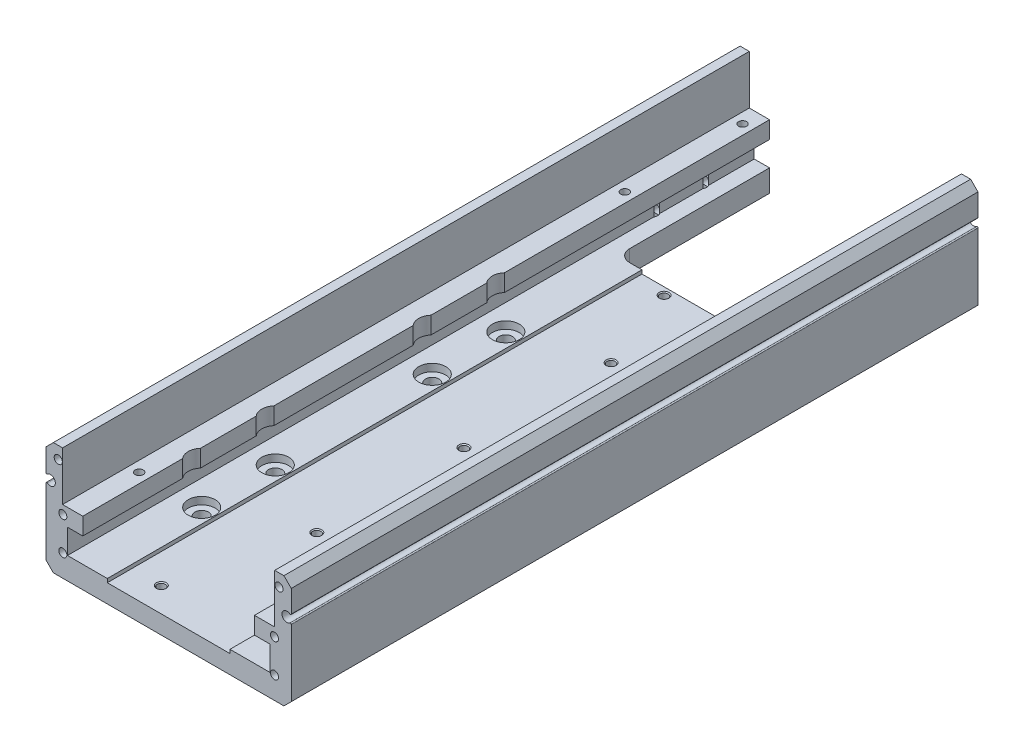
from build123d import *

# Parameters (mm, degrees)
SKETCH_1_W                          = 100
SKETCH_1_H                          = 46
EXTRUDE_1_DEPTH                     = 140
CHAMFER_1_SIZE                      = 3
CUT_EXTRUDE_1_DEPTH                 = 151.429385427
CUT_EXTRUDE_1_DEPTH_BACK            = 151.429385427
CUT_EXTRUDE_2_DEPTH                 = 151.429385427
CUT_EXTRUDE_2_DEPTH_BACK            = 151.429385427
SKETCH_3_R                          = 1.6
CUT_EXTRUDE_3_DEPTH                 = 151.429385427
CUT_EXTRUDE_3_DEPTH_BACK            = 151.429385427
SKETCH_4_R                          = 2
SKETCH_5_W                          = 70
SKETCH_5_H                          = 62
CUT_EXTRUDE_4_DEPTH                 = 156.614909311
HOLE_WIZARD_M4_1_AT_2_COUNT         = 2
HOLE_WIZARD_M4_1_AT_2_PITCH         = 32.053431954
HOLE_WIZARD_M4_1_AT_3_COUNT         = 2
HOLE_WIZARD_M4_1_AT_3_PITCH         = 93.77858231
HOLE_WIZARD_M4_1_AT_4_COUNT         = 2
HOLE_WIZARD_M4_1_AT_4_PITCH         = 86.3
FILLET_1_R                          = 5
HOLE_WIZARD_M4_2_REACH              = 152.917
HOLE_WIZARD_M4_2_BORE_R             = 1.65
FILLET_2_R                          = 0.35
HOLE_WIZARD_M5_1_D                  = 5.5
HOLE_WIZARD_M5_1_CBORE_D            = 11
HOLE_WIZARD_M5_1_CBORE_DEPTH        = 20
PATTERN_LINEAR_1_COUNT              = 2
PATTERN_LINEAR_1_PITCH              = 94
PATTERN_LINEAR_2_COUNT              = 2
PATTERN_LINEAR_2_PITCH              = 30
PATTERN_LINEAR_2_COPY_1_D           = 5.5
PATTERN_LINEAR_2_COPY_1_CBORE_D     = 11
PATTERN_LINEAR_2_COPY_1_CBORE_DEPTH = 20
SKETCH_17_R                         = 0.728078166
SKETCH_17_R_2                       = 0.853646628
SKETCH_17_R_3                       = 0.861040079
CUT_EXTRUDE_6_DEPTH                 = 33
SKETCH_18_R                         = 1.055541114
CUT_EXTRUDE_7_DEPTH                 = 33
HOLE_WIZARD_M4_5_D                  = 3.3
HOLE_WIZARD_M4_5_DEPTH              = 11.5
HOLE_WIZARD_M4_5_CSINK_D            = 4.05
HOLE_WIZARD_M4_5_CSINK_ANGLE        = 90
HOLE_WIZARD_M4_5_TIP                = 0.991420021
PATTERN_LINEAR_3_COUNT              = 2
PATTERN_LINEAR_3_PITCH              = 205
HOLE_WIZARD_M5_1_2_AT_2_COUNT       = 2
HOLE_WIZARD_M5_1_2_AT_2_PITCH       = 20


with BuildPart() as part:
    # 草图1 → 凸台-拉伸1 (new, symmetric)
    with BuildSketch(Plane.XY):
        Rectangle(SKETCH_1_W, SKETCH_1_H)
    extrude(amount=EXTRUDE_1_DEPTH, both=True)

    # 倒角1
    chamfer_1_edges = [part.edges().sort_by_distance(p)[0] for p in [
        (50, -23, 0),
        (-50, -23, 0),
        (-50, 23, 0),
        (50, 23, 0),
    ]]
    chamfer(chamfer_1_edges, length=CHAMFER_1_SIZE)

    # 草图2 → 切除-拉伸1 (cut, two sides: drawn at the far end of the back side and taken through both)
    with BuildSketch(Plane.XY.offset(-CUT_EXTRUDE_1_DEPTH_BACK)):
        Polygon((43.25, 23), (-43.25, 23), (-43.25, 3), (-35, 3), (-35, -4), (-41.25, -4), (-41.25, -14), (-25, -14), (-25, -15.5), (25, -15.5), (25, -14), (41.25, -14), (41.25, -4), (35, -4), (35, 3), (43.25, 3), align=None)
    extrude(amount=CUT_EXTRUDE_1_DEPTH + CUT_EXTRUDE_1_DEPTH_BACK, mode=Mode.SUBTRACT)

    # 草图3 → 切除-拉伸2 (cut, two sides: drawn at the far end of the back side and taken through both)
    with BuildSketch(Plane.XY.offset(-CUT_EXTRUDE_2_DEPTH_BACK)):
        with Locations((-43.15, -14)):
            Circle(SKETCH_3_R)
        with Locations((-45, 18)):
            Circle(SKETCH_3_R)
        with Locations(Location((43.15, -14, 0), (0, 0, 180))):
            Circle(SKETCH_3_R)
        with Locations(Location((45, 18, 0), (0, 0, 180))):
            Circle(SKETCH_3_R)
    extrude(amount=CUT_EXTRUDE_2_DEPTH + CUT_EXTRUDE_2_DEPTH_BACK, mode=Mode.SUBTRACT)

    # 草图4 → 切除-拉伸3 (cut, two sides: drawn at the far end of the back side and taken through both)
    with BuildSketch(Plane.XY.offset(-CUT_EXTRUDE_3_DEPTH_BACK)):
        with Locations((-48.2, 9.1)):
            Circle(SKETCH_4_R)
        with Locations((48.2, 9.1)):
            Circle(SKETCH_4_R)
    extrude(amount=CUT_EXTRUDE_3_DEPTH + CUT_EXTRUDE_3_DEPTH_BACK, mode=Mode.SUBTRACT)

    # 草图5 → 切除-拉伸4 (cut, through all)
    with BuildSketch(Plane.XZ.offset(23)):
        with Locations((0, -109)):
            Rectangle(SKETCH_5_W, SKETCH_5_H)
    extrude(amount=-CUT_EXTRUDE_4_DEPTH, mode=Mode.SUBTRACT)

    # 草图6 → M4 螺纹孔4 (revolve, cut)
    with BuildSketch(Plane(origin=(-43.15, -0.5, 140), x_dir=(0, -1, 0), z_dir=(1, 0, 0))):
        Polygon((0, 0), (0, 15.991420021), (1.65, 15), (1.65, 0), align=None)
    hole_wizard_m4_4 = revolve(axis=Axis((-43.15, -0.5, 146.35), (0, 0, -1)), mode=Mode.SUBTRACT)

    # 镜向1: M4 螺纹孔4 across plane
    add(hole_wizard_m4_4.mirror(Plane(origin=(0, 0, 0), x_dir=(0, 0, 1), z_dir=(1, 0, 0))), mode=Mode.SUBTRACT)

    # 镜向2: M4 螺纹孔4 across plane
    add(hole_wizard_m4_4.mirror(Plane.XY), mode=Mode.SUBTRACT)

    # 镜向2 copy 1 sketch → 镜向2 copy 1 (revolve, cut)
    with BuildSketch(Plane(origin=(43.15, -0.5, -140), x_dir=(0, -1, 0), z_dir=(-1, 0, 0))):
        Polygon((0, 0), (0, 15.991420021), (1.65, 15), (1.65, 0), align=None)
    revolve(axis=Axis((43.15, -0.5, -146.35), (0, 0, 1)), mode=Mode.SUBTRACT)

    # 草图8 → M4 螺纹孔1 (revolve, cut)
    with BuildSketch(Plane(origin=(-43.15, -14, 140), x_dir=(0, -1, 0), z_dir=(1, 0, 0))):
        Polygon((0, 0), (0, 12.991420021), (1.65, 12), (1.65, 0), align=None)
    hole_wizard_m4_1 = revolve(axis=Axis((-43.15, -14, 146.35), (0, 0, -1)), mode=Mode.SUBTRACT)

    # M4 螺纹孔1 at 2: M4 螺纹孔1 ×2
    with Locations(*[Vector(-0.05771612857810949, 0.9983330348645962, 0) * (i * HOLE_WIZARD_M4_1_AT_2_PITCH) for i in range(1, HOLE_WIZARD_M4_1_AT_2_COUNT)]):
        add(hole_wizard_m4_1, mode=Mode.SUBTRACT)

    # M4 螺纹孔1 at 3: M4 螺纹孔1 ×2
    with Locations(*[Vector(0.9399800874465586, 0.34122930003732144, 0) * (i * HOLE_WIZARD_M4_1_AT_3_PITCH) for i in range(1, HOLE_WIZARD_M4_1_AT_3_COUNT)]):
        add(hole_wizard_m4_1, mode=Mode.SUBTRACT)

    # M4 螺纹孔1 at 4: M4 螺纹孔1 ×2
    with Locations(*[(i * HOLE_WIZARD_M4_1_AT_4_PITCH, 0, 0) for i in range(1, HOLE_WIZARD_M4_1_AT_4_COUNT)]):
        add(hole_wizard_m4_1, mode=Mode.SUBTRACT)

    # 镜向3: M4 螺纹孔1 across plane
    add(hole_wizard_m4_1.mirror(Plane.XY), mode=Mode.SUBTRACT)

    # 镜向3 copy 1 sketch → 镜向3 copy 1 (revolve, cut)
    with BuildSketch(Plane(origin=(-45, 18, -140), x_dir=(0, -1, 0), z_dir=(1, 0, 0))):
        Polygon((0, 0), (0, -12.991420021), (1.65, -12), (1.65, 0), align=None)
    revolve(axis=Axis((-45, 18, -146.35), (0, 0, -1)), mode=Mode.SUBTRACT)

    # 镜向3 copy 2 sketch → 镜向3 copy 2 (revolve, cut)
    with BuildSketch(Plane(origin=(45, 18, -140), x_dir=(0, -1, 0), z_dir=(1, 0, 0))):
        Polygon((0, 0), (0, -12.991420021), (1.65, -12), (1.65, 0), align=None)
    revolve(axis=Axis((45, 18, -146.35), (0, 0, -1)), mode=Mode.SUBTRACT)

    # 镜向3 copy 3 sketch → 镜向3 copy 3 (revolve, cut)
    with BuildSketch(Plane(origin=(43.15, -14, -140), x_dir=(0, -1, 0), z_dir=(1, 0, 0))):
        Polygon((0, 0), (0, -12.991420021), (1.65, -12), (1.65, 0), align=None)
    revolve(axis=Axis((43.15, -14, -146.35), (0, 0, -1)), mode=Mode.SUBTRACT)

    # 圆角1
    fillet_1_edges = [part.edges().sort_by_distance(p)[0] for p in [
        (35, -18.5, -78),
        (-35, -18.5, -78),
    ]]
    fillet(fillet_1_edges, radius=FILLET_1_R)

    # M4 螺纹孔2 bore → M4 螺纹孔2 (cut, up to next)
    with BuildSketch(Plane(origin=(0, 3, 0), x_dir=(1, 0, 0), z_dir=(0, 1, 0)), mode=Mode.PRIVATE) as hole_wizard_m4_2_sk1:
        with Locations((-39, 133)):
            Circle(HOLE_WIZARD_M4_2_BORE_R)
    hole_wizard_m4_2_tool1 = extrude(hole_wizard_m4_2_sk1.sketch, amount=-HOLE_WIZARD_M4_2_REACH, mode=Mode.PRIVATE) & part.part
    # M4 螺纹孔2 bore → M4 螺纹孔2 (cut, up to next)
    with BuildSketch(Plane(origin=(0, 3, 0), x_dir=(1, 0, 0), z_dir=(0, 1, 0)), mode=Mode.PRIVATE) as hole_wizard_m4_2_sk2:
        with Locations((-39, 85)):
            Circle(HOLE_WIZARD_M4_2_BORE_R)
    hole_wizard_m4_2_tool2 = extrude(hole_wizard_m4_2_sk2.sketch, amount=-HOLE_WIZARD_M4_2_REACH, mode=Mode.PRIVATE) & part.part
    # M4 螺纹孔2 bore → M4 螺纹孔2 (cut, up to next)
    with BuildSketch(Plane(origin=(0, 3, 0), x_dir=(1, 0, 0), z_dir=(0, 1, 0)), mode=Mode.PRIVATE) as hole_wizard_m4_2_sk3:
        with Locations((-39, -113)):
            Circle(HOLE_WIZARD_M4_2_BORE_R)
    hole_wizard_m4_2_tool3 = extrude(hole_wizard_m4_2_sk3.sketch, amount=-HOLE_WIZARD_M4_2_REACH, mode=Mode.PRIVATE) & part.part
    hole_wizard_m4_2_1 = hole_wizard_m4_2_tool1.solids().sort_by_distance((-39, 3, -133))[0]
    add(hole_wizard_m4_2_1, mode=Mode.SUBTRACT)
    hole_wizard_m4_2_2 = hole_wizard_m4_2_tool2.solids().sort_by_distance((-39, 3, -85))[0]
    add(hole_wizard_m4_2_2, mode=Mode.SUBTRACT)
    hole_wizard_m4_2_3 = hole_wizard_m4_2_tool3.solids().sort_by_distance((-39, 3, 113))[0]
    add(hole_wizard_m4_2_3, mode=Mode.SUBTRACT)
    hole_wizard_m4_2 = hole_wizard_m4_2_1 + hole_wizard_m4_2_2 + hole_wizard_m4_2_3  # M4 螺纹孔2 as one shape, for the pattern or mirror that repeats it

    # 镜向4: M4 螺纹孔2 across plane
    add(hole_wizard_m4_2.mirror(Plane(origin=(0, 0, 0), x_dir=(0, 0, 1), z_dir=(1, 0, 0))), mode=Mode.SUBTRACT)

    # 圆角2
    fillet_2_edges = [part.edges().sort_by_distance(p)[0] for p in [
        (-50, 9.971779789, 0),
        (-50, 8.228220211, 0),
        (50, 8.228220211, 0),
        (50, 9.971779789, 0),
    ]]
    fillet(fillet_2_edges, radius=FILLET_2_R)

    # Hole Wizard M5 _1 (through all)
    with Locations(Plane(origin=(30.854497241, 3, -28.333612976), x_dir=(1, 0, 0), z_dir=(0, 1, 0))):
        with Locations((0, 0), (-61.708994482, 0)):
            hole_wizard_m5_1 = CounterBoreHole(HOLE_WIZARD_M5_1_D / 2, HOLE_WIZARD_M5_1_CBORE_D / 2, HOLE_WIZARD_M5_1_CBORE_DEPTH)

    # 阵列(线性)1: Hole Wizard M5 _1 ×2
    with Locations(*[(0, 0, i * PATTERN_LINEAR_1_PITCH) for i in range(1, PATTERN_LINEAR_1_COUNT)]):
        add(hole_wizard_m5_1, mode=Mode.SUBTRACT)

    # 阵列(线性)2: Hole Wizard M5 _1 ×2
    with Locations(*[(0, 0, i * PATTERN_LINEAR_2_PITCH) for i in range(1, PATTERN_LINEAR_2_COUNT)]):
        add(hole_wizard_m5_1, mode=Mode.SUBTRACT)

    # 阵列(线性)2 copy 1 (through all)
    with Locations(Plane(origin=(30.854497241, 3, 95.666387024), x_dir=(1, 0, 0), z_dir=(0, 1, 0))):
        with Locations((0, 0), (-61.708994482, 0)):
            CounterBoreHole(PATTERN_LINEAR_2_COPY_1_D / 2, PATTERN_LINEAR_2_COPY_1_CBORE_D / 2, PATTERN_LINEAR_2_COPY_1_CBORE_DEPTH)

    # 草图17 → 切除-拉伸6 (cut)
    with BuildSketch(Plane(origin=(0, -15.5, 0), x_dir=(1, 0, 0), z_dir=(0, 1, 0))):
        with Locations(Location((0, 40.4, 0), (0, 0, 180))):
            Circle(SKETCH_17_R)
        with Locations(Location((0, -79.6, 0), (0, 0, 180))):
            Circle(SKETCH_17_R_2)
        with Locations(Location((0, -19.6, 0), (0, 0, 180))):
            Circle(SKETCH_17_R_3)
    extrude(amount=-CUT_EXTRUDE_6_DEPTH, mode=Mode.SUBTRACT)

    # 草图18 → 切除-拉伸7 (cut)
    with BuildSketch(Plane(origin=(0, -15.5, 0), x_dir=(1, 0, 0), z_dir=(0, 1, 0))):
        with Locations(Location((-13, -130, 0), (0, 0, 180))):
            Circle(SKETCH_18_R)
    extrude(amount=-CUT_EXTRUDE_7_DEPTH, mode=Mode.SUBTRACT)

    # M4 螺纹孔5
    with Locations(Plane(origin=(0, -15.5, 79.6), x_dir=(1, 0, 0), z_dir=(0, 1, 0))):
        with Locations((0, 0), (0, 60), (0, 120)):
            CounterSinkHole(HOLE_WIZARD_M4_5_D / 2, HOLE_WIZARD_M4_5_CSINK_D / 2, depth=HOLE_WIZARD_M4_5_DEPTH, counter_sink_angle=HOLE_WIZARD_M4_5_CSINK_ANGLE)
            with Locations((0, 0, -(HOLE_WIZARD_M4_5_DEPTH + HOLE_WIZARD_M4_5_TIP / 2))):  # 118° drill point
                Cone(0, HOLE_WIZARD_M4_5_D / 2, HOLE_WIZARD_M4_5_TIP, mode=Mode.SUBTRACT)

    # 草图20 → M4 螺纹孔6 (revolve, cut)
    with BuildSketch(Plane(origin=(-13, -15.5, 130), x_dir=(0, 0, 1), z_dir=(1, 0, 0))):
        Polygon((0, 0), (0, 12.491420021), (1.65, 11.5), (1.65, 0.375), (2.025, 0), align=None)
    hole_wizard_m4_6 = revolve(axis=Axis((-13, -9.15, 130), (0, -1, 0)), mode=Mode.SUBTRACT)

    # 阵列(线性)3: M4 螺纹孔6 ×2
    with Locations(*[(0, 0, -i * PATTERN_LINEAR_3_PITCH) for i in range(1, PATTERN_LINEAR_3_COUNT)]):
        add(hole_wizard_m4_6, mode=Mode.SUBTRACT)

    # 草图22 → Hole Wizard M5 _1 2 (revolve, cut)
    with BuildSketch(Plane(origin=(43, -23, -120.264435853), x_dir=(0, 0, -1), z_dir=(1, 0, 0))):
        Polygon((0, 0), (0, 15.2618073), (2.1, 14), (2.1, 0), align=None)
    hole_wizard_m5_1_2 = revolve(axis=Axis((43, -29.35, -120.264435853), (0, 1, 0)), mode=Mode.SUBTRACT)

    # Hole Wizard M5 _1 2 at 2: Hole Wizard M5 _1 2 ×2
    with Locations(*[(0, 0, i * HOLE_WIZARD_M5_1_2_AT_2_PITCH) for i in range(1, HOLE_WIZARD_M5_1_2_AT_2_COUNT)]):
        add(hole_wizard_m5_1_2, mode=Mode.SUBTRACT)

    # 镜向5: Hole Wizard M5 _1 2 across plane
    add(hole_wizard_m5_1_2.mirror(Plane(origin=(0, 0, 0), x_dir=(0, 0, 1), z_dir=(1, 0, 0))), mode=Mode.SUBTRACT)

    # 镜向5 copy 1 sketch → 镜向5 copy 1 (revolve, cut)
    with BuildSketch(Plane(origin=(-43, -23, -100.264435853), x_dir=(0, 0, -1), z_dir=(-1, 0, 0))):
        Polygon((0, 0), (0, -15.2618073), (2.1, -14), (2.1, 0), align=None)
    revolve(axis=Axis((-43, -29.35, -100.264435853), (0, -1, 0)), mode=Mode.SUBTRACT)


solid = part.part
